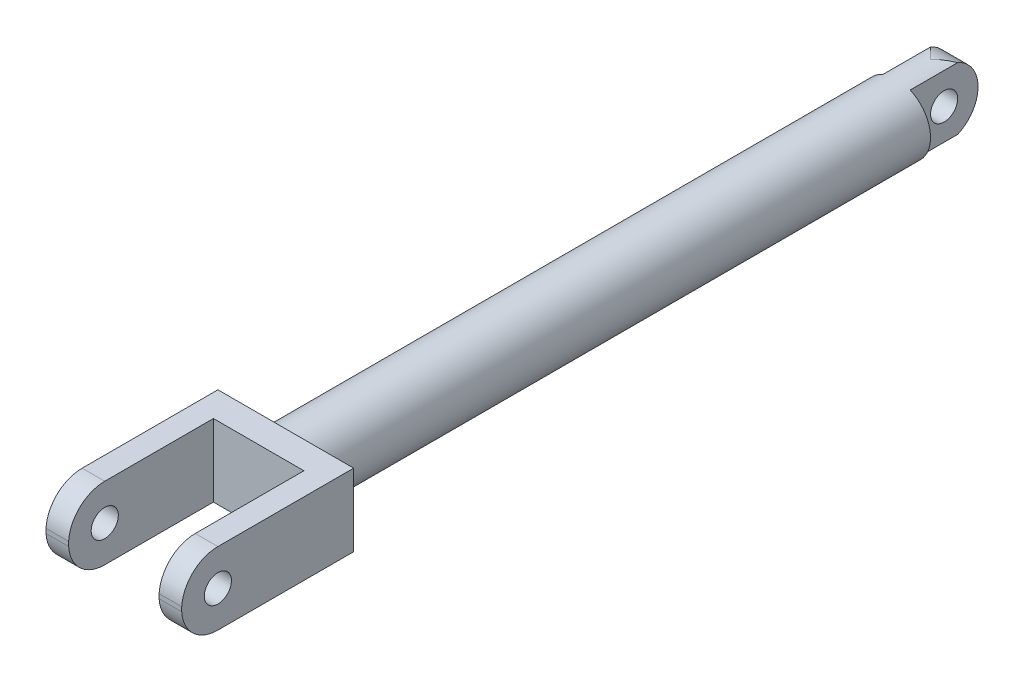
from build123d import *

# Parameters (mm, degrees)
SKETCH1_R               = 7.5
BOSS_EXTRUDE1_DEPTH     = 150
SKETCH2_W               = 30
SKETCH2_H               = 16
BOSS_EXTRUDE2_DEPTH     = 38
SKETCH3_W               = 20
SKETCH3_H               = 19.358131828
CUT_EXTRUDE1_DEPTH      = 32
CUT_EXTRUDE2_DEPTH      = 191.546582231
CUT_EXTRUDE2_DEPTH_BACK = 191.546582231
SKETCH4_R               = 3
CUT_EXTRUDE3_DEPTH      = 189.76705221
CUT_EXTRUDE3_DEPTH_BACK = 189.76705221
SKETCH5_W               = 4.5
SKETCH5_H               = 15
SKETCH5_W_2             = 19.942706309
CUT_EXTRUDE4_DEPTH      = 190.029098289
CUT_EXTRUDE4_DEPTH_BACK = 190.029098289
SKETCH6_R               = 3


with BuildPart() as part:
    # Sketch1 → Boss-Extrude1 (new body)
    with BuildSketch(Plane.XY):
        Circle(SKETCH1_R)
    extrude(amount=BOSS_EXTRUDE1_DEPTH)

    # Sketch2 → Boss-Extrude2 (add)
    with BuildSketch(Plane.XY.offset(150)):
        Rectangle(SKETCH2_W, SKETCH2_H)
    extrude(amount=BOSS_EXTRUDE2_DEPTH)

    # Sketch3 → Cut-Extrude1 (cut)
    with BuildSketch(Plane.XY.offset(188)):
        Rectangle(SKETCH3_W, SKETCH3_H)
    extrude(amount=-CUT_EXTRUDE1_DEPTH, mode=Mode.SUBTRACT)

    # Sketch4 → Cut-Extrude2 (cut, two sides: drawn at the far end of the back side and taken through both)
    with BuildSketch(Plane(origin=(15, 0, 0), x_dir=(0, 0, -1), z_dir=(1, 0, 0)).offset(-CUT_EXTRUDE2_DEPTH_BACK)):
        with Locations(Location((-180.014983451, 0, 0), (0, 0, 90))):
            Circle(SKETCH4_R)
        with BuildLine():
            Line((-180.014983451, 8), (-180.014983451, 17.706818894))
            Line((-180.014983451, 17.706818894), (-220.326825599, 17.706818894))
            Line((-220.326825599, 17.706818894), (-218.614105417, -20.299257523))
            Line((-218.614105417, -20.299257523), (-180.014983451, -8))
            ThreePointArc((-180.014983451, -8), (-188.014983451, 0), (-180.014983451, 8))
        make_face()
    extrude(amount=CUT_EXTRUDE2_DEPTH + CUT_EXTRUDE2_DEPTH_BACK, mode=Mode.SUBTRACT)

    # Sketch5 → Cut-Extrude3 (cut, two sides: drawn at the far end of the back side and taken through both)
    with BuildSketch(Plane(origin=(0, 0, 0), x_dir=(1, 0, 0), z_dir=(0, 1, 0)).offset(-CUT_EXTRUDE3_DEPTH_BACK)):
        with Locations((-5.25, -7.5)):
            Rectangle(SKETCH5_W, SKETCH5_H)
        with Locations((12.971353155, -7.5)):
            Rectangle(SKETCH5_W_2, SKETCH5_H)
    extrude(amount=CUT_EXTRUDE3_DEPTH + CUT_EXTRUDE3_DEPTH_BACK, mode=Mode.SUBTRACT)

    # Sketch6 → Cut-Extrude4 (cut, two sides: drawn at the far end of the back side and taken through both)
    with BuildSketch(Plane.ZY.offset(3).offset(-CUT_EXTRUDE4_DEPTH_BACK)):
        with Locations((7.5, 0)):
            Circle(SKETCH6_R)
        with BuildLine():
            Line((7.5, 7.5), (-1.727121044, 19.130973882))
            Line((-1.727121044, 19.130973882), (-13.960832092, -5.232772696))
            Line((-13.960832092, -5.232772696), (1.279468959, -23.272312715))
            Line((1.279468959, -23.272312715), (7.5, -7.5))
            ThreePointArc((7.5, -7.5), (0, 0), (7.5, 7.5))
        make_face()
    extrude(amount=CUT_EXTRUDE4_DEPTH + CUT_EXTRUDE4_DEPTH_BACK, mode=Mode.SUBTRACT)


solid = part.part
